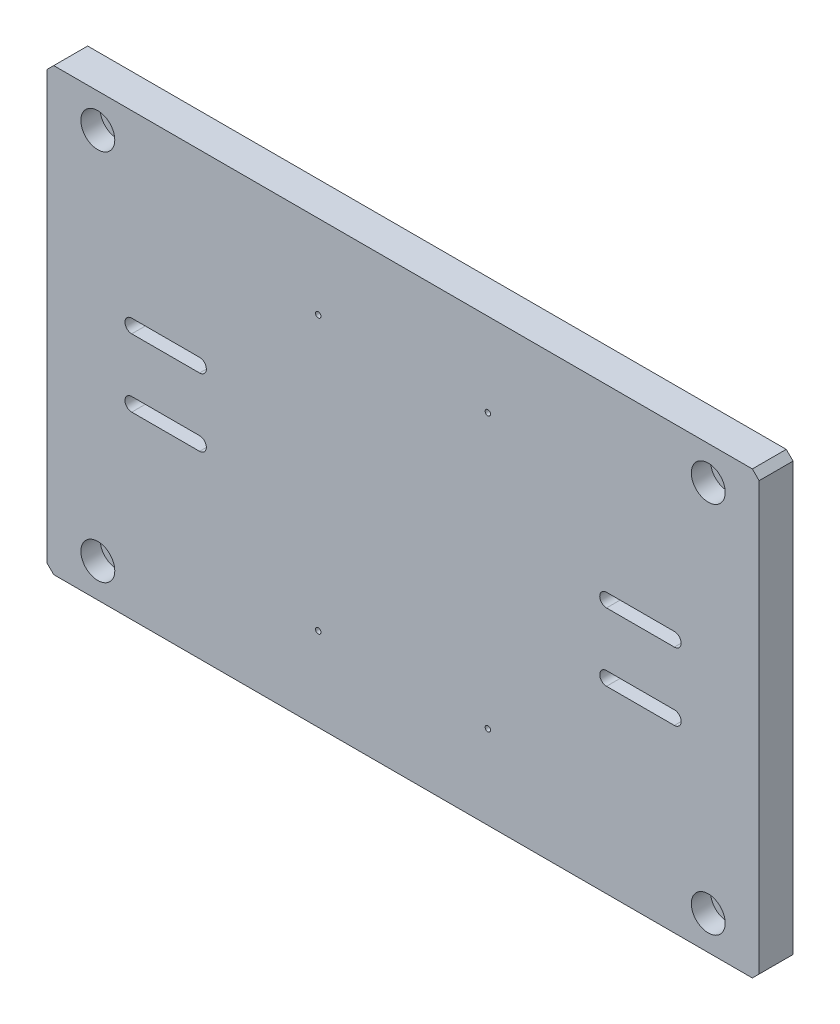
SolidWorks part; units mm, degrees
ref_plane "Front Plane" through (0, 0, 0) normal (0, 0, 1) x (1, 0, 0)
ref_plane "Top Plane" through (0, 0, 0) normal (0, 1, 0) x (1, 0, 0)
ref_plane "Right Plane" through (0, 0, 0) normal (1, 0, 0) x (0, 0, -1)
sketch "Sketch1" plane through (0, 0, 0) normal (0, 0, 1) x (1, 0, 0)
  line L1 (-105, -65) -> (105, -65)
  line L2 (-105, -65) -> (-105, 65)
  line L3 (-105, 65) -> (105, 65)
  line L4 (105, -65) -> (105, 65)
  line L5 (-105, -65) -> (105, 65) construction
  line L6 (-105, 65) -> (105, -65) construction
  point P0 (0, 0)
  dimension "D1" = 210
  dimension "D2" = 130
extrude "Boss-Extrude1" add sketch "Sketch1" along normal blind 10
sketch "Sketch2" plane through (0, 0, 10) normal (0, 0, 1) x (1, 0, 0)
  line L0 (-122.0076, 0) -> (116.5676, 0) construction
  line L1 (0, 81.5601) -> (0, -104.8714) construction
  line L2 (-80, 10) -> (-60, 10) construction
  line L3 (-80, 12) -> (-60, 12)
  line L4 (-80, 8) -> (-60, 8)
  line L5 (-30, 55) -> (-30, 25) construction
  line L8 (-28, 55) -> (-28, 25)
  line L9 (-32, 55) -> (-32, 25)
  line L11 (-80, -10) -> (-60, -10) construction
  line L12 (-80, -12) -> (-60, -12)
  line L13 (-80, -8) -> (-60, -8)
  line L14 (30, 55) -> (30, 25) construction
  line L15 (28, 55) -> (28, 25)
  line L16 (32, 55) -> (32, 25)
  line L17 (-30, -55) -> (-30, -25) construction
  line L18 (-28, -55) -> (-28, -25)
  line L19 (-32, -55) -> (-32, -25)
  line L20 (30, -55) -> (30, -25) construction
  line L21 (28, -55) -> (28, -25)
  line L22 (32, -55) -> (32, -25)
  line L23 (80, 10) -> (60, 10) construction
  line L24 (80, 12) -> (60, 12)
  line L25 (80, 8) -> (60, 8)
  line L26 (80, -10) -> (60, -10) construction
  line L27 (80, -12) -> (60, -12)
  line L28 (80, -8) -> (60, -8)
  arc A0 (-80, 12) -> (-80, 8) centre (-80, 10) ccw
  arc A1 (-60, 8) -> (-60, 12) centre (-60, 10) ccw
  arc A4 (-28, 55) -> (-32, 55) centre (-30, 55) ccw
  arc A5 (-32, 25) -> (-28, 25) centre (-30, 25) ccw
  arc A6 (-80, -12) -> (-80, -8) centre (-80, -10) cw
  arc A7 (-60, -8) -> (-60, -12) centre (-60, -10) cw
  arc A8 (28, 55) -> (32, 55) centre (30, 55) cw
  arc A9 (32, 25) -> (28, 25) centre (30, 25) cw
  arc A10 (-28, -55) -> (-32, -55) centre (-30, -55) cw
  arc A11 (-32, -25) -> (-28, -25) centre (-30, -25) cw
  arc A12 (28, -55) -> (32, -55) centre (30, -55) ccw
  arc A13 (32, -25) -> (28, -25) centre (30, -25) ccw
  arc A14 (80, 12) -> (80, 8) centre (80, 10) cw
  arc A15 (60, 8) -> (60, 12) centre (60, 10) cw
  arc A16 (80, -12) -> (80, -8) centre (80, -10) ccw
  arc A17 (60, -8) -> (60, -12) centre (60, -10) ccw
  point P7 (-70, 10)
  point P14 (-30, 40)
  point P21 (-70, -10)
  point P28 (30, 40)
  point P35 (-30, -40)
  point P42 (30, -40)
  point P49 (70, 10)
  point P56 (70, -10)
  dimension "D1" = 20
  dimension "D2" = 70
  dimension "D3" = 10
  dimension "D4" = 4
  dimension "D5" = 4
  dimension "D6" = 30
  dimension "D7" = 30
  dimension "D8" = 40
extrude "Cut-Extrude1" cut sketch "Sketch2" against normal through all both and the other way through all contours L4 A1 L3 A0 | A7 L13 A6 L12 | L28 A17 L27 A16 | L24 A15 L25 A14
sketch "Sketch3" plane through (0, 0, 10) normal (0, 0, 1) x (1, 0, 0)
  line L0 (-25, 40.35) -> (25, 40.35)
  line L1 (-90, 55) -> (90, 55)
  line L2 (-90, 55) -> (-90, -55)
  line L3 (-90, -55) -> (90, -55)
  line L4 (90, 55) -> (90, -55)
  line L5 (-25, -40.35) -> (25, -40.35)
hole_wizard "Hole size (per socket head cap screw type)1" positions "3DSketch1" profile "Sketch4" counterbore size "M5" standard "GB" end condition through all
sketch3d "3DSketch1"
  point P0 (-90, 55, 10)
  point P3 (-90, -55, 10)
  point P6 (90, -55, 10)
  point P9 (90, 55, 10)
sketch "Sketch4" plane through (-90, 55, 10) normal (1, 0, 0) x (0, -1, 0)
  line L0 (0, 0) -> (0, 10)
  line L1 (0, 10) -> (2.75, 10)
  line L3 (2.75, 10) -> (2.75, 5.7)
  line L4 (2.75, 5.7) -> (5, 5.7)
  line L5 (5, 5.7) -> (5, 0)
  line L7 (5, 0) -> (0, 0)
  line L11 (0, -6.35) -> (0, 107.95) construction
  dimension "通孔孔直径" = 5.5
  dimension "通孔孔深度" = 10
  dimension "柱形沉头孔直径" = 10
  dimension "柱形沉头孔深度" = 5.7
hole_wizard "M2 Tapped Hole1" positions "3DSketch3" profile "Sketch6" tap size "M2" standard "GB" end condition through all
sketch3d "3DSketch3"
  point P0 (-25, 40.35, 10)
  point P3 (25, 40.35, 10)
  point P6 (25, -40.35, 10)
  point P9 (-25, -40.35, 10)
sketch "Sketch6" plane through (-25, 40.35, 10) normal (1, 0, 0) x (0, -1, 0)
  line L0 (0, 0) -> (0, 10)
  line L1 (0, 10) -> (0.8, 10)
  line L2 (0.8, 10) -> (0.8, 0)
  line L5 (0.8, 0) -> (0, 0)
  line L11 (0, -6.35) -> (0, 107.95) construction
  dimension "通孔螺纹孔钻头直径" = 1.6
  dimension "通孔螺纹孔钻头深度" = 10
cosmetic thread "Cosmetic thread1" parameters "D2"=2
cosmetic thread "Cosmetic thread2" parameters "D2"=2
cosmetic thread "Cosmetic thread3" parameters "D2"=2
cosmetic thread "Cosmetic thread4" parameters "D2"=2
chamfer "Chamfer1" distance 2 angle 45 4 edges at (-105, 65, 5) (-105, -65, 5) (105, -65, 5) (105, 65, 5)
